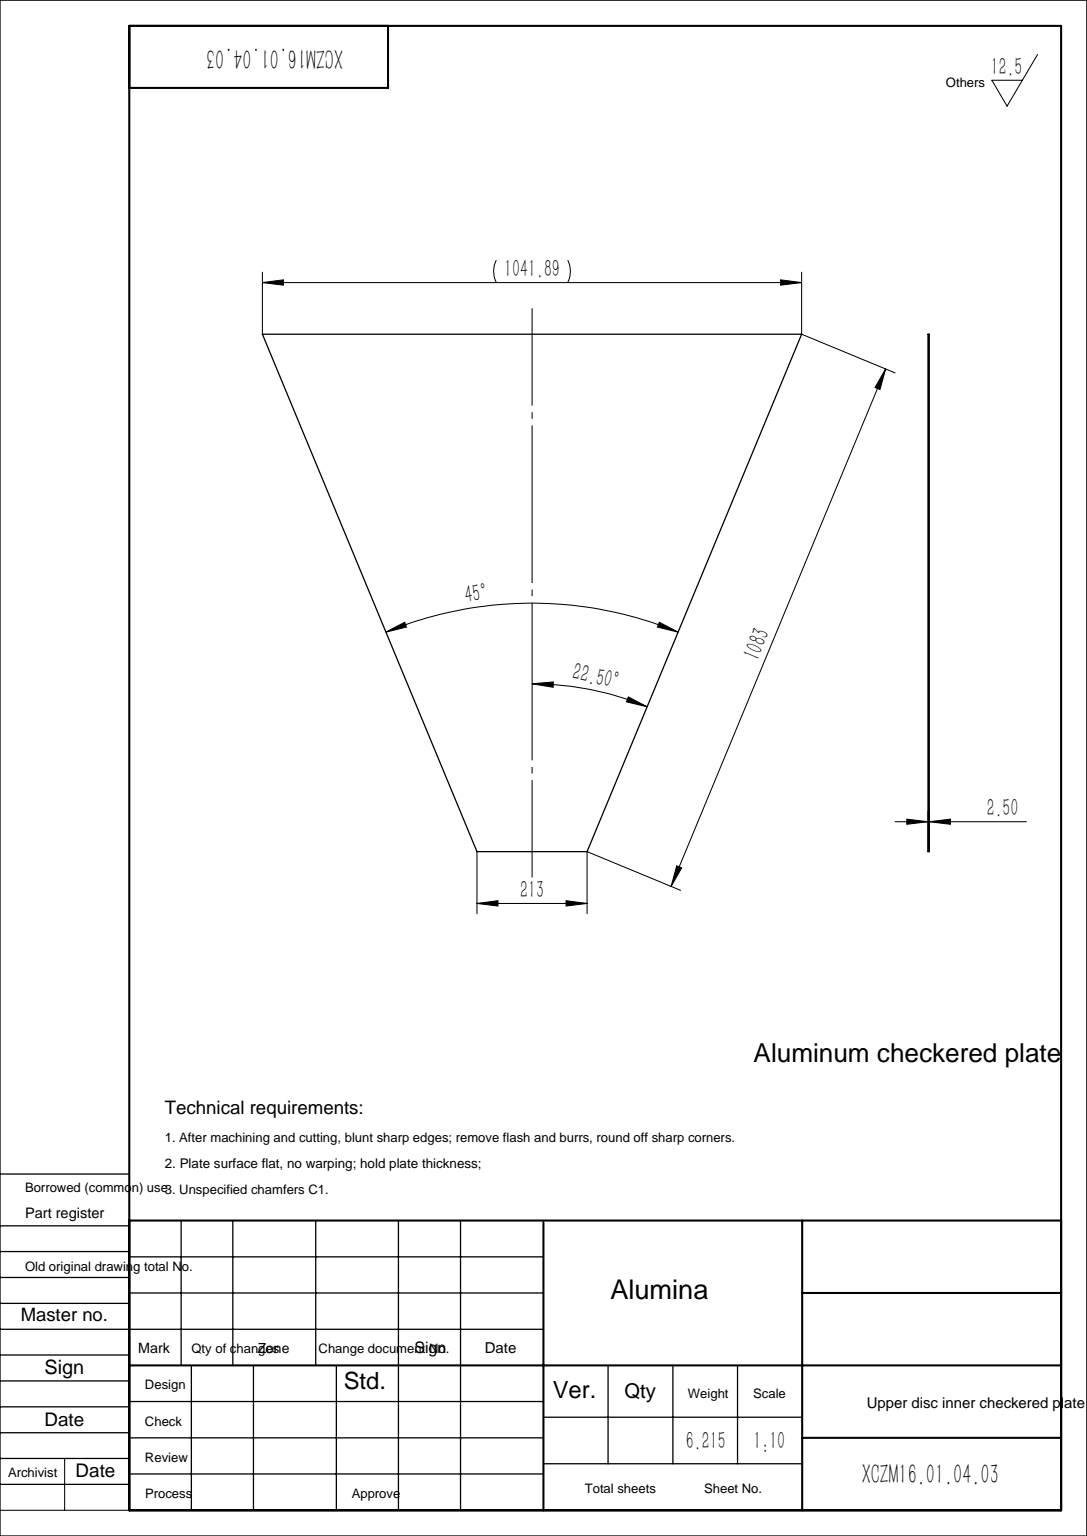
from build123d import *

# Parameters (mm, degrees)
BOSS_EXTRUDE1_DEPTH = 2.5


with BuildPart() as part:
    # Sketch1 → Boss-Extrude1 (new body)
    with BuildSketch(Plane.XY):
        Polygon((0, 1000.56153371), (0, 0), (106.5, 0), (520.946157251, 1000.56153371), align=None)
        Polygon((-106.5, 0), (0, 0), (0, 1000.56153371), (-520.946157251, 1000.56153371), align=None)
    extrude(amount=BOSS_EXTRUDE1_DEPTH)


solid = part.part
